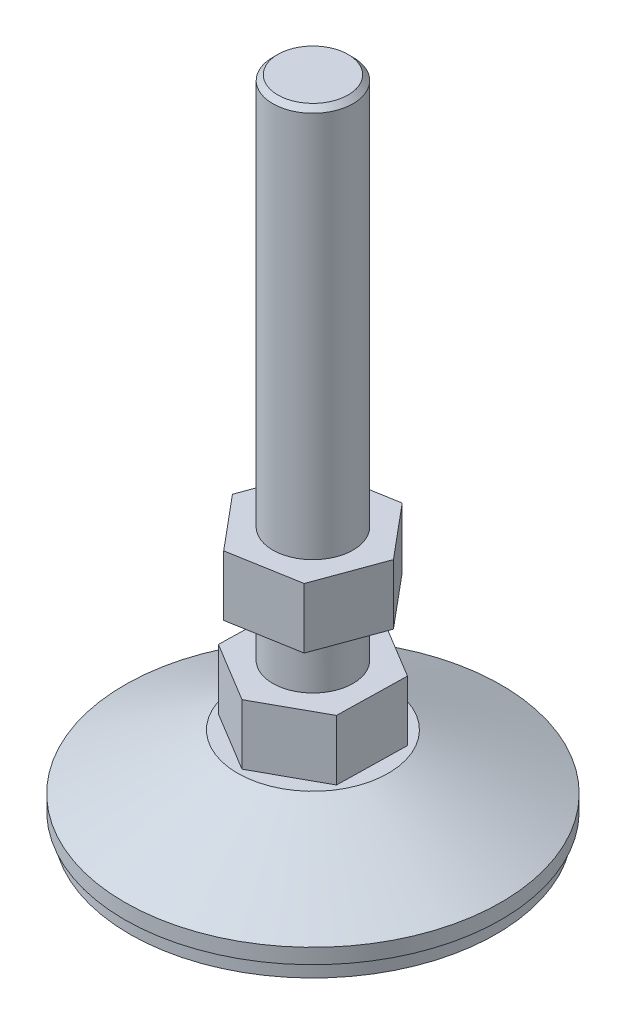
from build123d import *

# Parameters (mm, degrees)
EXTRUDE1_DEPTH = 12
EXTRUDE2_START = 35
EXTRUDE2_DEPTH = 12
CHAMFER1_SIZE  = 1


with BuildPart() as part:
    # Sketch1 → Revolve1 (revolve)
    with BuildSketch(Plane.XY, mode=Mode.PRIVATE) as revolve1_sk:
        Polygon((-37.5, 10.372678427), (-15, 21.372678427), (-8, 21.372678427), (-8, 134.372678427), (0, 134.372678427), (0, 4.372678427), (-36.5, 4.372678427), (-36.5, 7.372678427), (-37.5, 7.372678427), align=None)
    revolve(revolve1_sk.sketch.rotate(Axis((0, 0, 0), (0, -1, 0)), 270), axis=Axis((0, 0, 0), (0, -1, 0)))

    # Sketch2 → Extrude1 (add)
    with BuildSketch(Plane(origin=(0, 21.372678427, 0), x_dir=(-1, 0, 0), z_dir=(0, 1, 0))):
        Polygon((-11.859328821, 7.166332389), (-12.135890312, -6.687313836), (-0.27656149, -13.853646226), (11.859328821, -7.166332389), (12.135890312, 6.687313836), (0.27656149, 13.853646226), align=None)
    extrude(amount=EXTRUDE1_DEPTH)

    # Sketch3 → Extrude2 (add)
    with BuildSketch(Plane(origin=(0, 21.372678427, 0), x_dir=(-1, 0, 0), z_dir=(0, 1, 0)).offset(EXTRUDE2_START)):
        Polygon((-8.887785091, 10.63048805), (-13.650165251, -2.381803647), (-4.76238016, -13.012291697), (8.887785091, -10.63048805), (13.650165251, 2.381803647), (4.76238016, 13.012291697), align=None)
    extrude(amount=-EXTRUDE2_DEPTH)

    # Chamfer1
    chamfer1_edges = [part.edges().sort_by_distance(p)[0] for p in [
        (0, 134.372678427, -8),
    ]]
    chamfer(chamfer1_edges, length=CHAMFER1_SIZE)


solid = part.part
